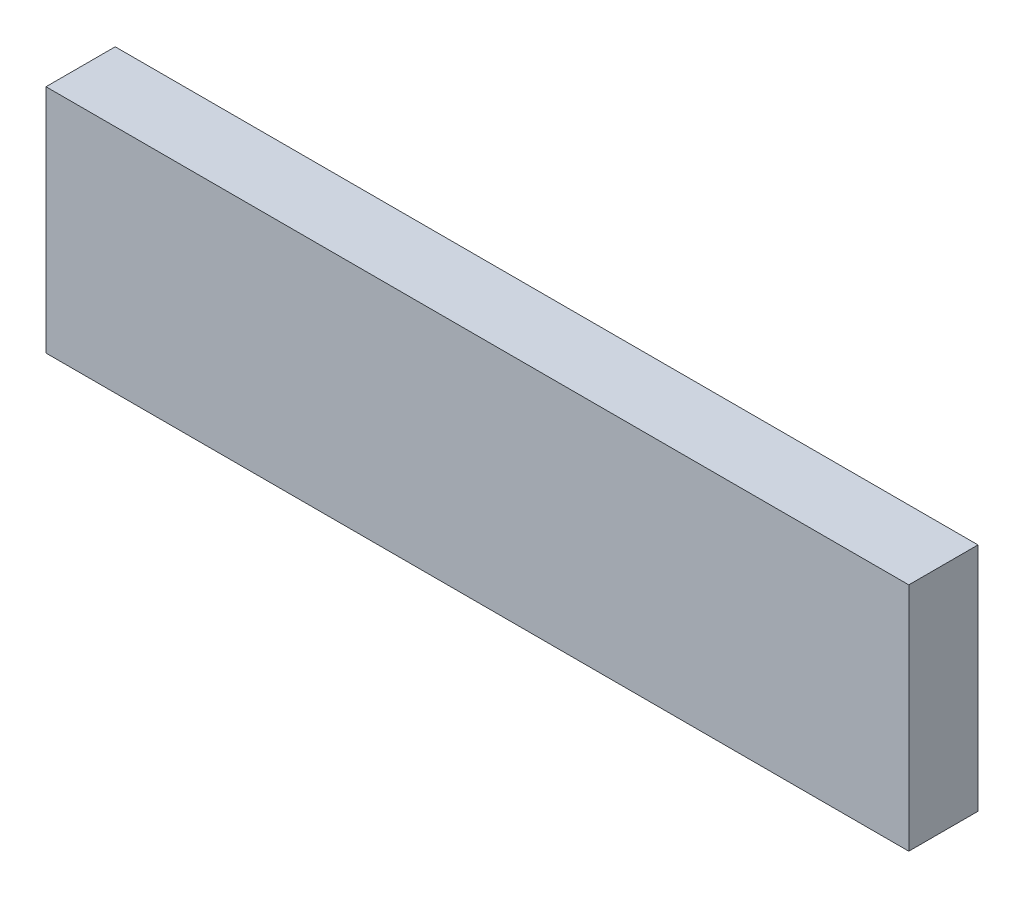
from build123d import *

# Parameters (mm, degrees)
SKETCH_1_W      = 187
SKETCH_1_H      = 50
EXTRUDE_1_DEPTH = 15


with BuildPart() as part:
    # 草图1 → 凸台-拉伸1 (new body)
    with BuildSketch(Plane.XY):
        Rectangle(SKETCH_1_W, SKETCH_1_H)
    extrude(amount=EXTRUDE_1_DEPTH)


solid = part.part
